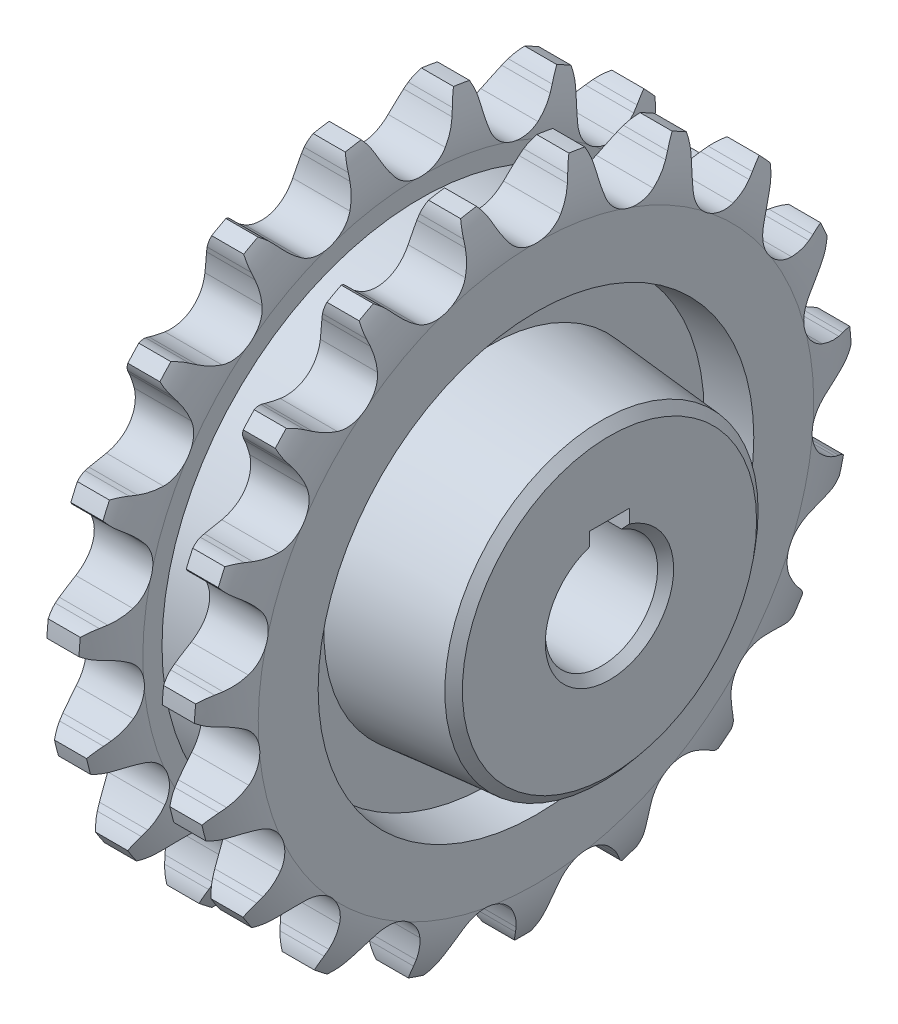
from build123d import *
from OCP.BRepFilletAPI import BRepFilletAPI_MakeChamfer

# Parameters (mm, degrees)
CUT_EXTRUDE1_DEPTH = 5.475375
CIRPATTERN1_COUNT  = 19
LPATTERN1_COUNT    = 2
LPATTERN1_PITCH    = 14.38
CHAMFER1_SIZE      = 1
CHAMFER1_SIZE2     = 1.100062868
SKETCH4_W          = 5
SKETCH4_H          = 2.761651585
CUT_EXTRUDE4_DEPTH = 71.401283385


with BuildPart() as part:
    # Sketch1 → Revolve1 (revolve)
    with BuildSketch(Plane.XY, mode=Mode.PRIVATE) as revolve1_sk:
        with BuildLine():
            Line((-3.65025, 27.149639763), (-3.65025, 34.619639763))
            ThreePointArc((-3.65025, 34.619639763), (-3.245836945, 37.918781526), (-1.99925, 41))
            Line((-1.99925, 41), (1.99925, 41))
            ThreePointArc((1.99925, 41), (3.245836945, 37.918781526), (3.65025, 34.619639763))
            Line((3.65025, 34.619639763), (3.65025, 27.149639763))
            Line((3.65025, 27.149639763), (-3.65025, 27.149639763))
        make_face()
    revolve(revolve1_sk.sketch.rotate(Axis((-6.35, 0, 0), (1, 0, 0)), 90), axis=Axis((-6.35, 0, 0), (1, 0, 0)))

    # Sketch2 → Cut-Extrude1 (cut, symmetric)
    with BuildSketch(Plane(origin=(0, 0, 0), x_dir=(0, 0, -1), z_dir=(1, 0, 0))):
        with BuildLine():
            Line((4.552244709, 38.426451297), (4.858741585, 39.1448403))
            ThreePointArc((4.858741585, 39.1448403), (5.250930322, 39.90290393), (5.750855114, 40.594675334))
            ThreePointArc((5.750855114, 40.594675334), (0, 41), (-5.750855114, 40.594675334))
            ThreePointArc((-5.750855114, 40.594675334), (-5.250930322, 39.90290393), (-4.858741585, 39.1448403))
            Line((-4.858741585, 39.1448403), (-4.552244709, 38.426451297))
            ThreePointArc((-4.552244709, 38.426451297), (-3.937302758, 37.212676935), (-3.168676608, 36.089905522))
            ThreePointArc((-3.168676608, 36.089905522), (0, 34.549839763), (3.168676608, 36.089905522))
            ThreePointArc((3.168676608, 36.089905522), (3.937302758, 37.212676935), (4.552244709, 38.426451297))
        make_face()
    cut_extrude1 = extrude(amount=CUT_EXTRUDE1_DEPTH, both=True, mode=Mode.SUBTRACT)

    # CirPattern1: Cut-Extrude1 ×19 about axis
    cirpattern1_axis = Axis((0, 0, 0), (1, 0, 0))
    for i in range(1, CIRPATTERN1_COUNT):
        add(cut_extrude1.rotate(cirpattern1_axis, i * 360 / CIRPATTERN1_COUNT), mode=Mode.SUBTRACT)


with BuildPart() as lpattern1_1:
    # LPattern1: pattern copy
    add(part.part.moved(Location(Vector(1, 0, 0) * (1 * LPATTERN1_PITCH))))


with BuildPart() as part_1:
    add(part.part)

    # Sketch5 → Revolve2 (revolve)
    with BuildSketch(Plane.XY, mode=Mode.PRIVATE) as revolve2_sk:
        Polygon((-12.81, 7), (27.19, 7), (27.19, 19.438259462), (12.34, 20.737466115), (12.34, 26.651807396), (18.03025, 27.149639763), (10.72975, 32.229639763), (3.65025, 32.229639763), (-3.65025, 27.149639763), (2.04, 26.651807396), (2.04, 20.737466115), (-12.81, 19.438259462), align=None)
    revolve(revolve2_sk.sketch.rotate(Axis((0, 0, 0), (-1, 0, 0)), 90), axis=Axis((0, 0, 0), (-1, 0, 0)))

    # Chamfer1: one chamfer whose edges measure the first distance from different faces: ONE call of the kernel's chamfer builder (chamfer() names one face for all edges)
    chamfer1_edges_1 = [part_1.edges().sort_by_distance(p)[0] for p in [
        (-12.81, 0, 7),
        (27.19, 0, 7),
    ]]
    chamfer1_edges_2 = [part_1.edges().sort_by_distance(p)[0] for p in [
        (-12.81, 0, 19.438259462),
    ]]
    chamfer1_side_2 = [part_1.faces().sort_by_distance(p)[0] for p in [
        (-12.81, 0, 18.888462459),
    ]]
    chamfer1_edges_3 = [part_1.edges().sort_by_distance(p)[0] for p in [
        (27.19, 0, 19.438259462),
    ]]
    chamfer1_side_3 = [part_1.faces().sort_by_distance(p)[0] for p in [
        (19.765, 0, 20.087862789),
    ]]
    chamfer1 = BRepFilletAPI_MakeChamfer(part_1.part.solid().wrapped)
    for e in chamfer1_edges_1:
        chamfer1.Add(CHAMFER1_SIZE, e.wrapped)
    for e in chamfer1_edges_2:
        chamfer1.Add(CHAMFER1_SIZE, CHAMFER1_SIZE2, e.wrapped, chamfer1_side_2[0].wrapped)  # the first distance lies on this face
    for e in chamfer1_edges_3:
        chamfer1.Add(CHAMFER1_SIZE, CHAMFER1_SIZE2, e.wrapped, chamfer1_side_3[0].wrapped)  # the first distance lies on this face
    add(Compound.cast(chamfer1.Shape()), mode=Mode.REPLACE)

    # Sketch4 → Cut-Extrude4 (cut, through all)
    with BuildSketch(Plane.ZY.offset(12.81)):
        with Locations((0, 7.919174208)):
            Rectangle(SKETCH4_W, SKETCH4_H)
    extrude(amount=-CUT_EXTRUDE4_DEPTH, mode=Mode.SUBTRACT)


solid = Compound([lpattern1_1.part, part_1.part])
